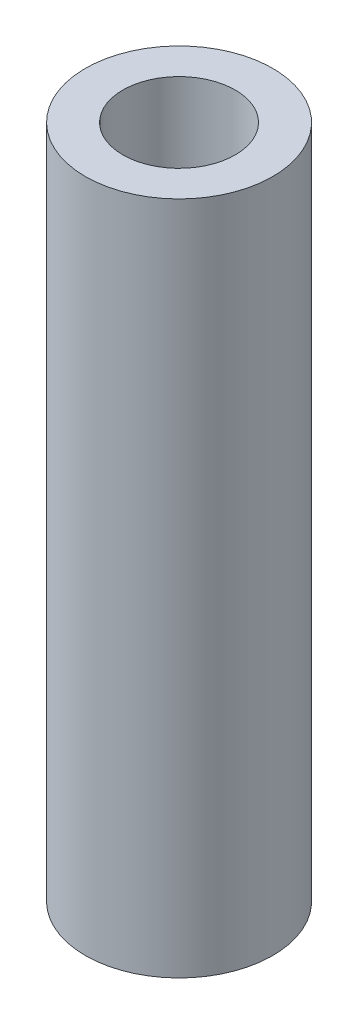
SolidWorks part; units mm, degrees
material "6061 合金"
ref_plane "前视基准面" through (0, 0, 0) normal (0, 0, 1) x (1, 0, 0)
ref_plane "上视基准面" through (0, 0, 0) normal (0, 1, 0) x (1, 0, 0)
ref_plane "右视基准面" through (0, 0, 0) normal (1, 0, 0) x (0, 0, -1)
other "Configuration Table"
sketch "草图1" plane through (0, 0, 0) normal (0, 1, 0) x (1, 0, 0)
  circle A0 centre (0, 0) radius 1.5
  circle A1 centre (0, 0) radius 2.5
  dimension "D1" = 3
  dimension "D2" = 5
extrude "凸台-拉伸1" add sketch "草图1" along normal blind 18
